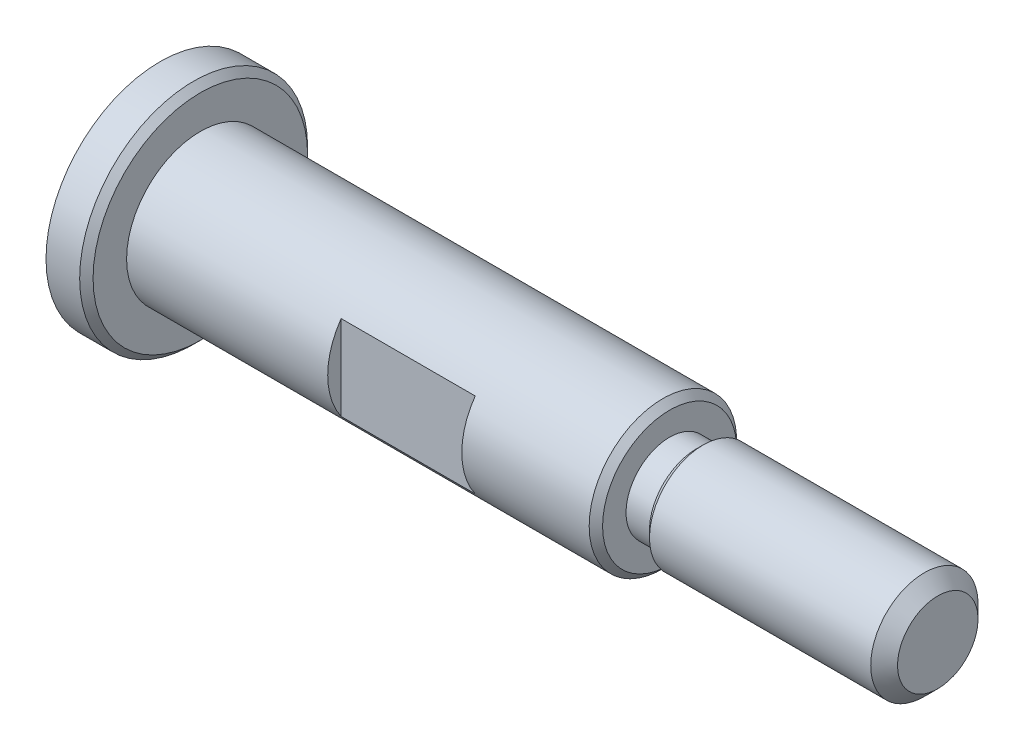
from build123d import *

# Parameters (mm, degrees)
SKETCH2_W          = 10
SKETCH2_H          = 1
CUT_EXTRUDE2_DEPTH = 5
CHAMFER1_SIZE      = 0.5
SKETCH3_W          = 2
SKETCH3_H          = 0.75
CHAMFER2_SIZE      = 0.5


with BuildPart() as part:
    # Sketch1 → Revolve1 (revolve)
    with BuildSketch(Plane.XY, mode=Mode.PRIVATE) as revolve1_sk:
        with BuildLine():
            Line((59.5, 3), (58.5, 4))
            Line((58.5, 4), (39.5, 4))
            Line((39.5, 4), (39.5, 5.5))
            Line((39.5, 5.5), (4.5, 5.5))
            Line((4.5, 5.5), (4.5, 8.5))
            Line((4.5, 8.5), (1.489364109, 8.5))
            ThreePointArc((1.489364109, 8.5), (0.375155866, 4.314748123), (0, 0))
            Line((0, 0), (59.5, 0))
            Line((59.5, 0), (59.5, 3))
        make_face()
    revolve(revolve1_sk.sketch.rotate(Axis((0, 0, 0), (1, 0, 0)), 90), axis=Axis((0, 0, 0), (1, 0, 0)))

    # Sketch2 → Cut-Extrude2 (cut, symmetric)
    with BuildSketch(Plane(origin=(0, 0, 0), x_dir=(1, 0, 0), z_dir=(0, 1, 0))):
        with Locations((24.5, 5)):
            Rectangle(SKETCH2_W, SKETCH2_H)
    cut_extrude2 = extrude(amount=CUT_EXTRUDE2_DEPTH, both=True, mode=Mode.SUBTRACT)

    # Mirror1: Cut-Extrude2 across plane
    add(cut_extrude2.mirror(Plane.XY), mode=Mode.SUBTRACT)

    # Chamfer1
    chamfer1_edges = [part.edges().sort_by_distance(p)[0] for p in [
        (4.5, 0, -8.5),
        (39.5, 0, -5.5),
    ]]
    chamfer(chamfer1_edges, length=CHAMFER1_SIZE)

    # Sketch3 → Cut-Revolve1 (revolve, cut)
    with BuildSketch(Plane(origin=(0, 0, 0), x_dir=(1, 0, 0), z_dir=(0, 1, 0)), mode=Mode.PRIVATE) as cut_revolve1_sk:
        with Locations((40.5, 3.625)):
            Rectangle(SKETCH3_W, SKETCH3_H)
    revolve(cut_revolve1_sk.sketch.rotate(Axis((58.5, 0, 0), (-1, 0, 0)), 270), axis=Axis((58.5, 0, 0), (-1, 0, 0)), mode=Mode.SUBTRACT)

    # Chamfer2
    chamfer2_edges = [part.edges().sort_by_distance(p)[0] for p in [
        (41.5, 0, -4),
    ]]
    chamfer(chamfer2_edges, length=CHAMFER2_SIZE)


solid = part.part
